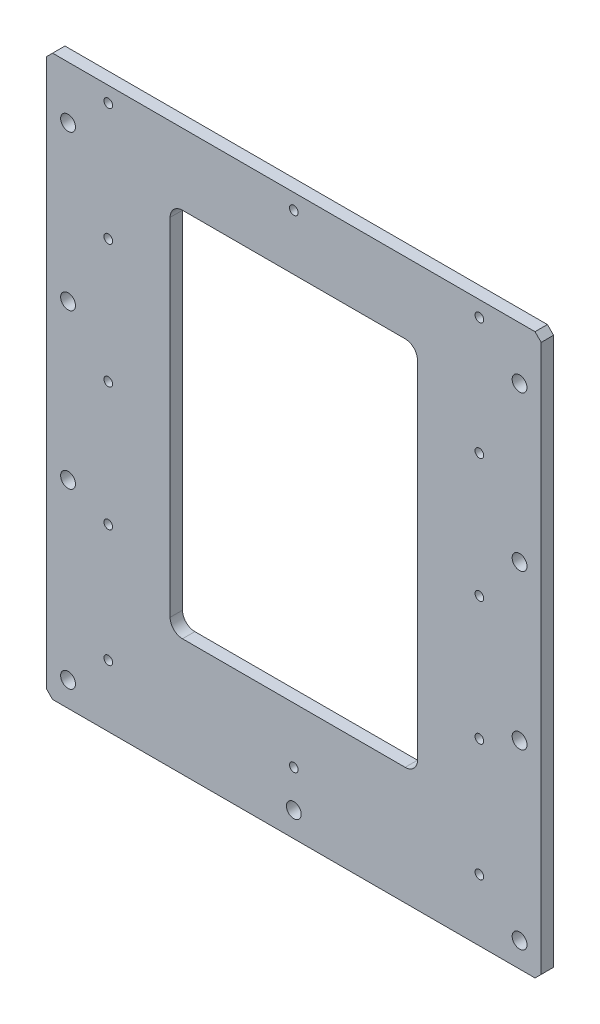
from build123d import *

# Parameters (mm, degrees)
SKETCH_1_W              = 800
SKETCH_1_H              = 980
EXTRUDE_1_DEPTH         = 20
HOLE_WIZARD_M16_1_D     = 14
HOLE_WIZARD_M16_1_DEPTH = 42
HOLE_WIZARD_M16_1_TIP   = 4.206024333
SKETCH_4_W              = 400
SKETCH_4_H              = 600
CUT_EXTRUDE_1_DEPTH     = 20
FILLET_1_R              = 20
SKETCH_10_W             = 800
SKETCH_10_H             = 75
CUT_EXTRUDE_3_DEPTH     = 633.850693292
HOLE_WIZARD_24_0_24_1_D = 24
CHAMFER_1_SIZE          = 10


with BuildPart() as part:
    # 草图1 → 凸台-拉伸1 (new body)
    with BuildSketch(Plane.XY):
        Rectangle(SKETCH_1_W, SKETCH_1_H)
    extrude(amount=EXTRUDE_1_DEPTH)

    # M16 螺纹孔1
    with Locations(Plane.XY.offset(20)):
        with Locations((300, 390), (-300, -390), (-300, 390), (300, -390), (-300, 0), (0, -390), (300, 0), (0, 390), (-300, 200), (300, 200), (-300, -200), (300, -200)):
            Hole(HOLE_WIZARD_M16_1_D / 2, depth=HOLE_WIZARD_M16_1_DEPTH)
            with Locations((0, 0, -(HOLE_WIZARD_M16_1_DEPTH + HOLE_WIZARD_M16_1_TIP / 2))):  # 118° drill point
                Cone(0, HOLE_WIZARD_M16_1_D / 2, HOLE_WIZARD_M16_1_TIP, mode=Mode.SUBTRACT)

    # 草图4 → 切除-拉伸1 (cut)
    with BuildSketch(Plane.XY.offset(20)):
        Rectangle(SKETCH_4_W, SKETCH_4_H)
    extrude(amount=-CUT_EXTRUDE_1_DEPTH, mode=Mode.SUBTRACT)

    # 圆角1
    fillet_1_edges = [part.edges().sort_by_distance(p)[0] for p in [
        (200, 300, 10),
        (200, -300, 10),
        (-200, -300, 10),
        (-200, 300, 10),
    ]]
    fillet(fillet_1_edges, radius=FILLET_1_R)

    # 草图10 → 切除-拉伸3 (cut, through all)
    with BuildSketch(Plane.XY.offset(20)):
        with Locations((0, 452.5)):
            Rectangle(SKETCH_10_W, SKETCH_10_H)
    extrude(amount=-CUT_EXTRUDE_3_DEPTH, mode=Mode.SUBTRACT)

    # Ø24.0 (24) 直径孔1 (through all)
    with Locations(Plane.XY.offset(20)):
        with Locations((365, 80), (365, -450), (-365, -450), (0, -450), (0, 450), (-365, 330), (365, 330), (-365, 80), (-365, -170), (365, -170)):
            Hole(HOLE_WIZARD_24_0_24_1_D / 2)

    # 倒角1
    chamfer_1_edges = [part.edges().sort_by_distance(p)[0] for p in [
        (-400, 415, 10),
        (400, 415, 10),
        (400, -490, 10),
        (-400, -490, 10),
    ]]
    chamfer(chamfer_1_edges, length=CHAMFER_1_SIZE)


solid = part.part
